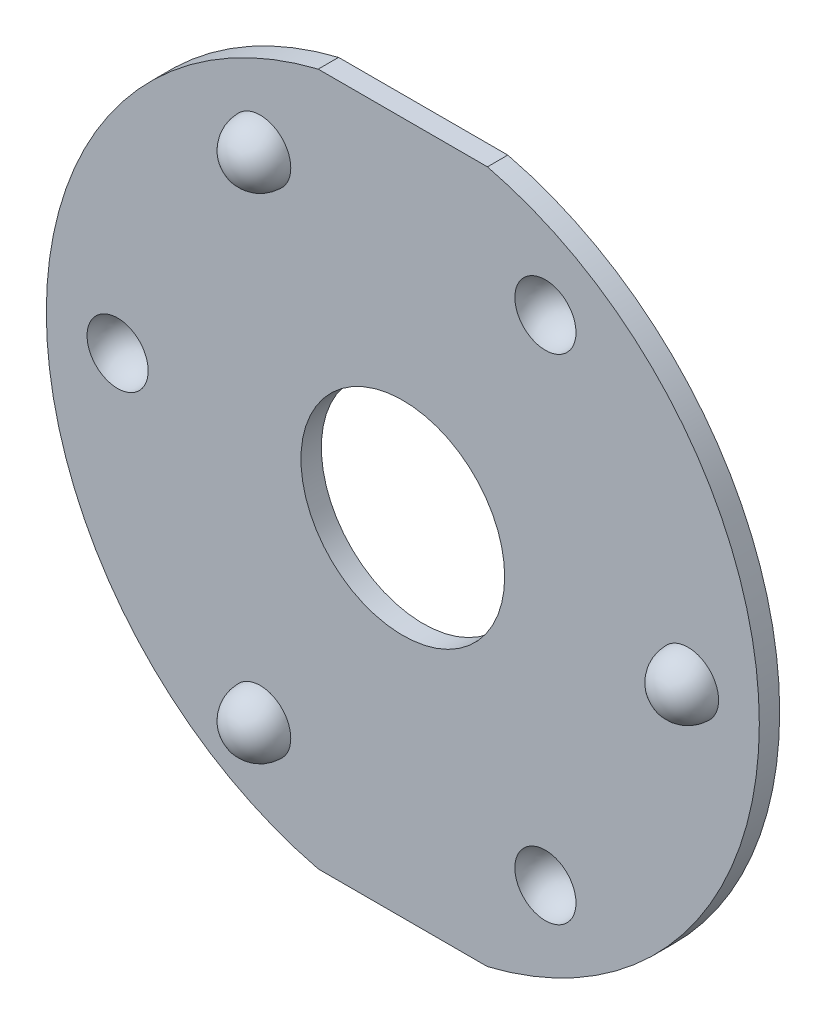
SolidWorks part; units mm, degrees
material "1.4000 (X6Cr13)"
ref_plane "Front Plane" through (0, 0, 0) normal (0, 0, 1) x (1, 0, 0)
ref_plane "Top Plane" through (0, 0, 0) normal (0, 1, 0) x (1, 0, 0)
ref_plane "Right Plane" through (0, 0, 0) normal (1, 0, 0) x (0, 0, -1)
sketch "Sketch1" plane through (0, 0, 0) normal (0, 0, 1) x (1, 0, 0)
  circle A0 centre (0, 0) radius 17.5
  circle A1 centre (0, 0) radius 5
  dimension "D1" = 35
  dimension "D2" = 10
extrude "Boss-Extrude1" add sketch "Sketch1" along normal mid plane 1
sketch "Sketch2" plane through (0, 0, 0.5) normal (0, 0, 1) x (1, 0, 0)
  line L0 (0, 0) -> (23.0533, 0) construction
  line L2 (-12.6154, 28.3022) -> (12.6154, 28.3022)
  line L3 (-12.6154, 28.3022) -> (-12.6154, 17)
  line L4 (-12.6154, 17) -> (12.6154, 17)
  line L5 (12.6154, 28.3022) -> (12.6154, 17)
  line L6 (-12.6154, 28.3022) -> (12.6154, 17) construction
  line L7 (-12.6154, 17) -> (12.6154, 28.3022) construction
  line L8 (-12.6154, -17) -> (12.6154, -17)
  line L9 (-12.6154, -17) -> (-12.6154, -27.8246)
  line L10 (-12.6154, -27.8246) -> (12.6154, -27.8246)
  line L11 (12.6154, -17) -> (12.6154, -27.8246)
  line L12 (-12.6154, -17) -> (12.6154, -27.8246) construction
  line L13 (-12.6154, -27.8246) -> (12.6154, -17) construction
  point P3 (0, 22.6511)
  point P8 (0, -22.4123)
  dimension "D1" = 17
  dimension "D2" = 17
extrude "Cut-Extrude1" cut sketch "Sketch2" against normal blind 1
sketch "Sketch3" plane through (0, 0, 0.5) normal (0, 0, 1) x (1, 0, 0)
  line L0 (0, 0) -> (14, 0) construction
  line L1 (14, 1.5) -> (14, -1.5) construction
  line L2 (14, 1.5) -> (14, -1.5)
  arc A0 (14, -1.5) -> (14, 1.5) centre (14, 0) ccw
  dimension "D2" = 3
  dimension "D1" = 14
revolve "Revolve1" add sketch "Sketch3" angle 360 about L2
pattern_circular "CirPattern1" count 3 over 360 about axis through (0, 0, 0) along (0, 0, 1) of "Revolve1"
sketch "Sketch4" plane through (0, 0, 0.5) normal (0, 0, 1) x (1, 0, 0)
  line L0 (0, 0) -> (-14, 0) construction
  line L1 (-14, 1.5) -> (-14, -1.5)
  arc A0 (-14, 1.5) -> (-14, -1.5) centre (-14, 0) ccw
  dimension "D2" = 3
  dimension "D1" = 14
sketch "Sketch5" plane through (0, 0, -0.5) normal (0, 0, -1) x (-1, 0, 0)
  line L0 (0, 0) -> (14, 0) construction
  line L1 (14, -1.5) -> (14, 1.5)
  arc A0 (14, -1.5) -> (14, 1.5) centre (14, 0) ccw
revolve "Revolve2" add sketch "Sketch5" angle 360 about L1
pattern_circular "CirPattern2" count 3 over 360 about axis through (0, 0, 0) along (0, 0, 1) of "Revolve2"
sketch "Sketch6" plane through (0, 0, 0.5) normal (0, 0, 1) x (1, 0, 0)
  line L0 (-14, 1.5) -> (-14, -1.5)
  arc A0 (-14, 1.5) -> (-14, -1.5) centre (-14, 0) ccw
revolve "Cut-Revolve2" cut sketch "Sketch6" angle 360 about L0
pattern_circular "CirPattern3" count 3 over 360 about axis through (0, 0, 0) along (0, 0, 1) of "Cut-Revolve2"
sketch "Sketch7" plane through (0, 0, -0.5) normal (0, 0, -1) x (-1, 0, 0)
  line L0 (-14, -1.118) -> (-14, 1.118)
  arc A1 (-14, 1.118) -> (-14, -1.118) centre (-14, 0) ccw
revolve "Cut-Revolve3" cut sketch "Sketch7" angle 360 about L0
pattern_circular "CirPattern4" count 3 over 360 about axis through (0, 0, 0) along (0, 0, 1) of "Cut-Revolve3"
